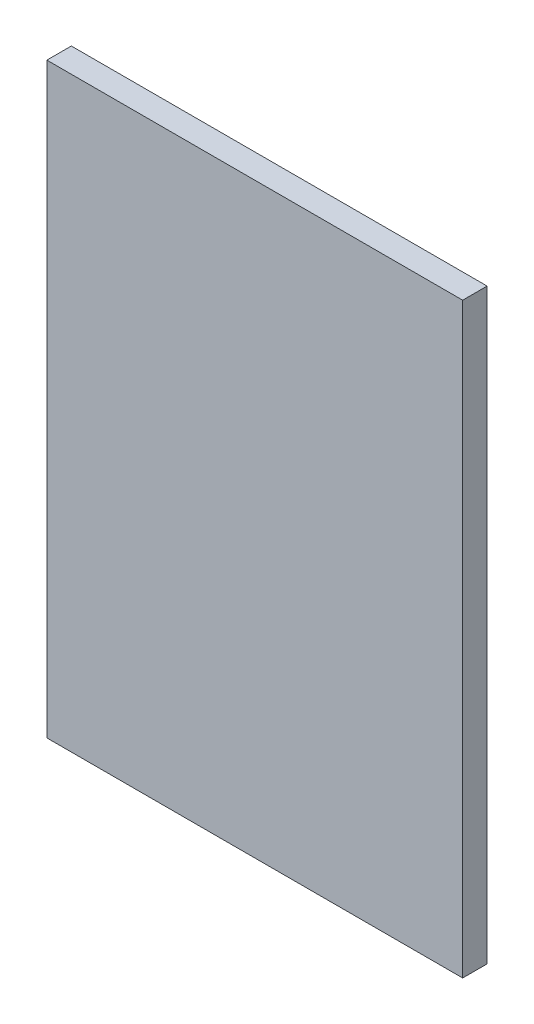
from build123d import *

# Parameters (mm, degrees)
SKETCH_1_W      = 170
SKETCH_1_H      = 240
EXTRUDE_1_DEPTH = 10


with BuildPart() as part:
    # 草图1 → 凸台-拉伸1 (new body)
    with BuildSketch(Plane.XY):
        Rectangle(SKETCH_1_W, SKETCH_1_H)
    extrude(amount=EXTRUDE_1_DEPTH)


solid = part.part
